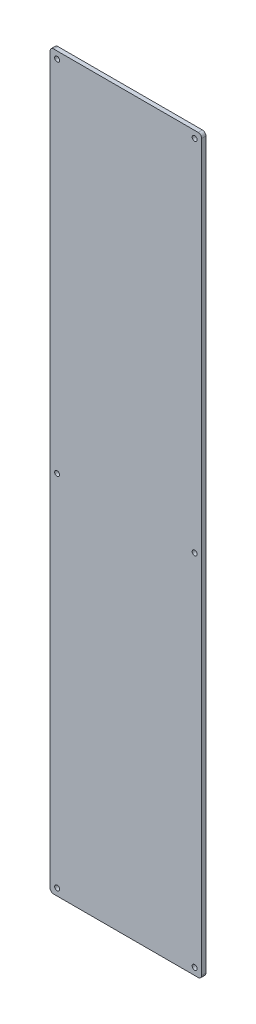
SolidWorks part; units mm, degrees
material "茶色亚克力"
ref_plane "前视基准面" through (0, 0, 0) normal (0, 0, 1) x (1, 0, 0)
ref_plane "上视基准面" through (0, 0, 0) normal (0, 1, 0) x (1, 0, 0)
ref_plane "右视基准面" through (0, 0, 0) normal (1, 0, 0) x (0, 0, -1)
sketch "草图1" plane through (0, 0, 0) normal (0, 0, 1) x (1, 0, 0)
  line L1 (-107.5, 519) -> (107.5, 519)
  line L2 (-107.5, 519) -> (-107.5, -519)
  line L3 (-107.5, -519) -> (107.5, -519)
  line L4 (107.5, 519) -> (107.5, -519)
  line L5 (-107.5, 519) -> (107.5, -519) construction
  line L6 (-107.5, -519) -> (107.5, 519) construction
  point P0 (0, 0)
  dimension "D1" = 215
  dimension "D2" = 1038
extrude "凸台-拉伸1" add sketch "草图1" along normal blind 6
hole_wizard "Ø7.0 (7) 直径孔1" positions "草图2" profile "草图3" hole size "Ø7.0" standard "GB" end condition through all
sketch "草图2" plane through (0, 0, 0) normal (0, 0, -1) x (-1, 0, 0)
  line L0 (0, 0) -> (0, 208.2434) construction
  line L3 (0, 0) -> (149.8874, 0) construction
  line L6 (-107.5, -519) -> (-107.5, 519) construction
  line L7 (-107.5, 519) -> (107.5, 519) construction
  point P0 (-97.5, 509)
  point P2 (-97.5, -509)
  point P4 (97.5, 509)
  point P6 (97.5, -509)
  point P28 (-97.5, 0)
  point P30 (97.5, 0)
  dimension "D1" = 10
  dimension "D2" = 10
sketch "草图3" plane through (97.5, 509, 0) normal (1, 0, 0) x (0, 1, 0)
  line L0 (0, 0) -> (0, 6)
  line L1 (0, 6) -> (3.5, 6)
  line L2 (3.5, 6) -> (3.5, 0)
  line L5 (3.5, 0) -> (0, 0)
  line L11 (0, -6.35) -> (0, 107.95) construction
  dimension "通孔孔直径" = 7
  dimension "通孔孔深度" = 6
fillet "圆角1" radius 5 4 edges at (-107.5, -519, 3) (-107.5, 519, 3) (107.5, -519, 3) (107.5, 519, 3)
